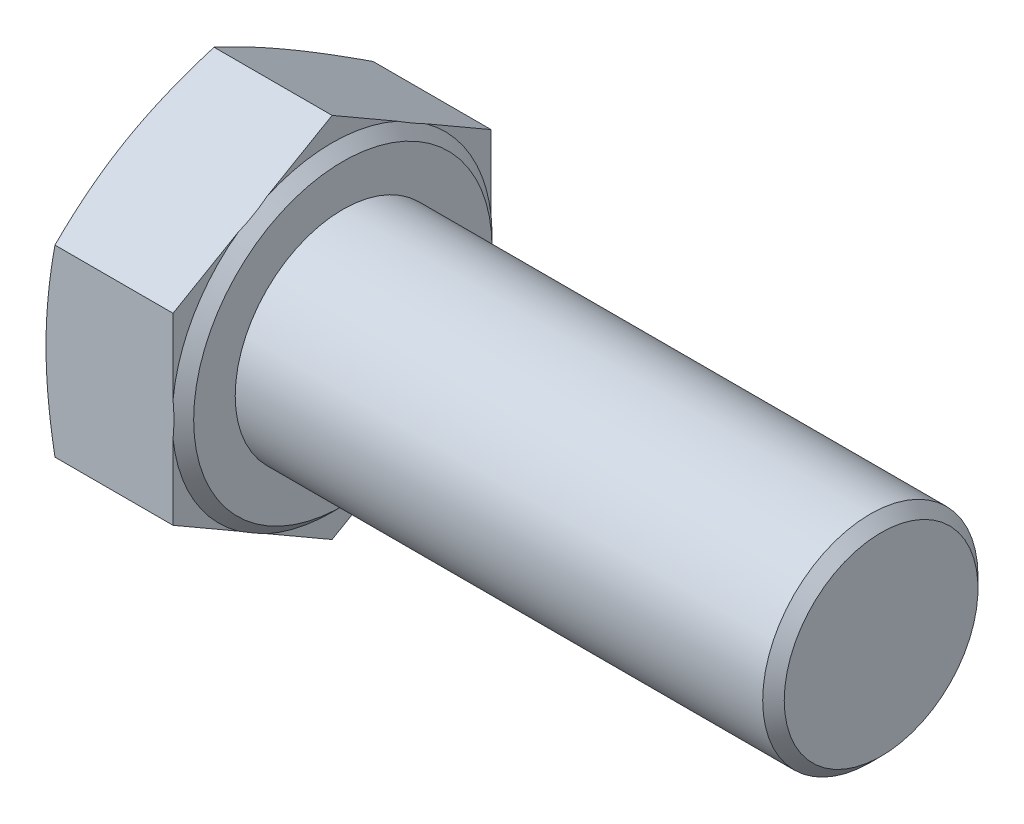
from build123d import *

# Parameters (mm, degrees)
BASEHEAD_DEPTH = 7.68
SKETCH5_R      = 6
BASEBODY_DEPTH = 30
CHAMFER1_SIZE  = 0.6


with BuildPart() as part:
    # Sketch2 → BaseHead (new body)
    with BuildSketch(Plane(origin=(0, 0, 0), x_dir=(0, 0, -1), z_dir=(1, 0, 0))):
        Polygon((8.865, -5.118210136), (8.865, 5.118210136), (0, 10.236420273), (-8.865, 5.118210136), (-8.865, -5.118210136), (0, -10.236420273), align=None)
    extrude(amount=BASEHEAD_DEPTH)

    # Sketch3 → BearingFace (revolve, cut)
    with BuildSketch(Plane.XY, mode=Mode.PRIVATE) as bearingface_sk:
        Polygon((7.68, 10.236420273), (7.68, 8.315), (7.08, 8.915), (7.08, 10.236420273), align=None)
    revolve(bearingface_sk.sketch.rotate(Axis((-0.957090588, 0, 0), (1, 0, 0)), 90), axis=Axis((-0.957090588, 0, 0), (1, 0, 0)), mode=Mode.SUBTRACT)

    # Sketch4 → HeadChamfer (revolve, cut)
    with BuildSketch(Plane.XY):
        Polygon((0, 10.236420273), (0.499156158, 10.236420273), (0, 8.865), align=None)
    revolve(axis=Axis((-0.493528746, 0, 0), (1, 0, 0)), mode=Mode.SUBTRACT)

    # Sketch5 → BaseBody (add)
    with BuildSketch(Plane(origin=(7.68, 0, 0), x_dir=(0, 0, -1), z_dir=(1, 0, 0))):
        Circle(SKETCH5_R)
    extrude(amount=BASEBODY_DEPTH)

    # Chamfer1
    chamfer1_edges = [part.edges().sort_by_distance(p)[0] for p in [
        (37.68, 0, 6),
    ]]
    chamfer(chamfer1_edges, length=CHAMFER1_SIZE)


solid = part.part
